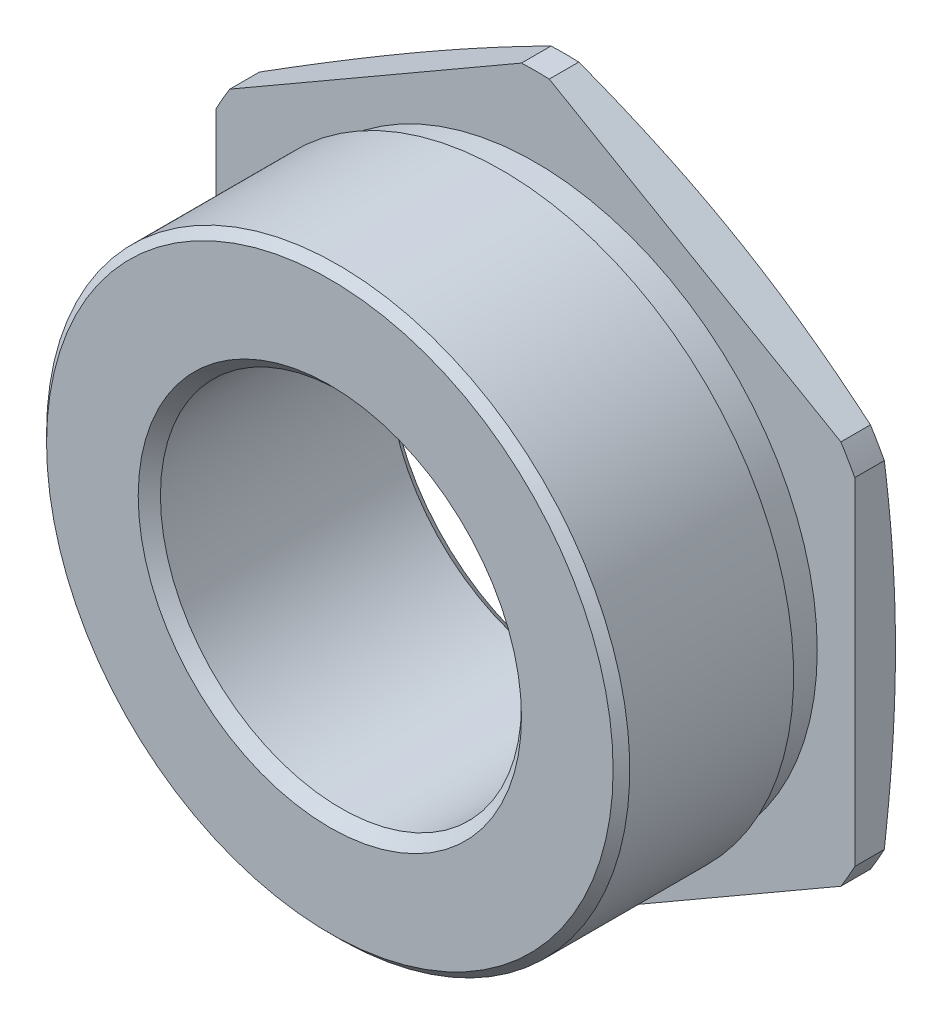
from build123d import *

# Parameters (mm, degrees)
BOSS_EXTRUDE1_DEPTH = 8
SKETCH2_R           = 52.5
BOSS_EXTRUDE2_DEPTH = 45
SKETCH3_R           = 52.5
SKETCH3_R_2         = 50.75
CUT_EXTRUDE1_DEPTH  = 6
SKETCH4_R           = 32.5
CUT_EXTRUDE2_DEPTH  = 98.75607398
CHAMFER1_SIZE       = 2
CHAMFER2_SIZE       = 1.5
SKETCH5_OUTSIDE_W   = 889.986
SKETCH5_OUTSIDE_H   = 904.986
SKETCH5_OUTSIDE_R   = 55
CUT_EXTRUDE3_DEPTH  = 98.75607398
CUT_EXTRUDE3_DRAFT  = -75


with BuildPart() as part:
    # Sketch1 → Boss-Extrude1 (new body)
    with BuildSketch(Plane.XY):
        with BuildLine():
            ThreePointArc((-2.5, -64.951905284), (0, -65), (2.5, -64.951905284))
            Line((2.5, -64.951905284), (55, -34.641016151))
            ThreePointArc((55, -34.641016151), (56.291651246, -32.5), (57.5, -30.310889132))
            Line((57.5, -30.310889132), (57.5, 30.310889132))
            ThreePointArc((57.5, 30.310889132), (56.291651246, 32.5), (55, 34.641016151))
            Line((55, 34.641016151), (2.5, 64.951905284))
            ThreePointArc((2.5, 64.951905284), (0, 65), (-2.5, 64.951905284))
            Line((-2.5, 64.951905284), (-55, 34.641016151))
            ThreePointArc((-55, 34.641016151), (-56.291651246, 32.5), (-57.5, 30.310889132))
            Line((-57.5, 30.310889132), (-57.5, -30.310889132))
            ThreePointArc((-57.5, -30.310889132), (-56.291651246, -32.5), (-55, -34.641016151))
            Line((-55, -34.641016151), (-2.5, -64.951905284))
        make_face()
    extrude(amount=BOSS_EXTRUDE1_DEPTH)

    # Sketch2 → Boss-Extrude2 (add)
    with BuildSketch(Plane(origin=(0, 0, 0), x_dir=(-1, 0, 0), z_dir=(0, 0, -1))):
        Circle(SKETCH2_R)
    extrude(amount=-BOSS_EXTRUDE2_DEPTH)

    # Sketch3 → Cut-Extrude1 (cut)
    with BuildSketch(Plane.XY.offset(8)):
        with Locations(Location((0, 0, 0), (0, 0, 180))):
            Circle(SKETCH3_R)
        Circle(SKETCH3_R_2, mode=Mode.SUBTRACT)
    extrude(amount=CUT_EXTRUDE1_DEPTH, mode=Mode.SUBTRACT)

    # Sketch4 → Cut-Extrude2 (cut, through all)
    with BuildSketch(Plane.XY.offset(45)):
        Circle(SKETCH4_R)
    extrude(amount=-CUT_EXTRUDE2_DEPTH, mode=Mode.SUBTRACT)

    # Chamfer1
    chamfer1_edges = [part.edges().sort_by_distance(p)[0] for p in [
        (-32.5, 0, 0),
        (-32.5, 0, 45),
    ]]
    chamfer(chamfer1_edges, length=CHAMFER1_SIZE)

    # Chamfer2
    chamfer2_edges = [part.edges().sort_by_distance(p)[0] for p in [
        (52.5, 0, 45),
    ]]
    chamfer(chamfer2_edges, length=CHAMFER2_SIZE)


with BuildPart() as cut_extrude3_tool:
    # Sketch5 outside → Cut-Extrude3 (with draft: the straight prism first)
    with BuildSketch(Plane(origin=(0, 0, 0), x_dir=(-1, 0, 0), z_dir=(0, 0, -1))):
        Rectangle(SKETCH5_OUTSIDE_W, SKETCH5_OUTSIDE_H)
        Circle(SKETCH5_OUTSIDE_R, mode=Mode.SUBTRACT)
    extrude(amount=-CUT_EXTRUDE3_DEPTH)
    # Cut-Extrude3: the draft: its side faces are tilted about the plane it starts from
    cut_extrude3_sides = [cut_extrude3_tool.faces().sort_by_distance(p)[0] for p in [
        (0, -452.493, 49.37803699),
        (-444.993, 0, 49.37803699),
        (0, 452.493, 49.37803699),
        (444.993, 0, 49.37803699),
        (55, 0, 49.37803699),
    ]]
    draft(cut_extrude3_sides, Plane(origin=(0, 0, 0), x_dir=(-1, 0, 0), z_dir=(0, 0, -1)), CUT_EXTRUDE3_DRAFT)


with BuildPart() as part_1:
    add(part.part)

    # Cut-Extrude3: cut by cut_extrude3_tool
    add(cut_extrude3_tool.part, mode=Mode.SUBTRACT)


solid = part_1.part
